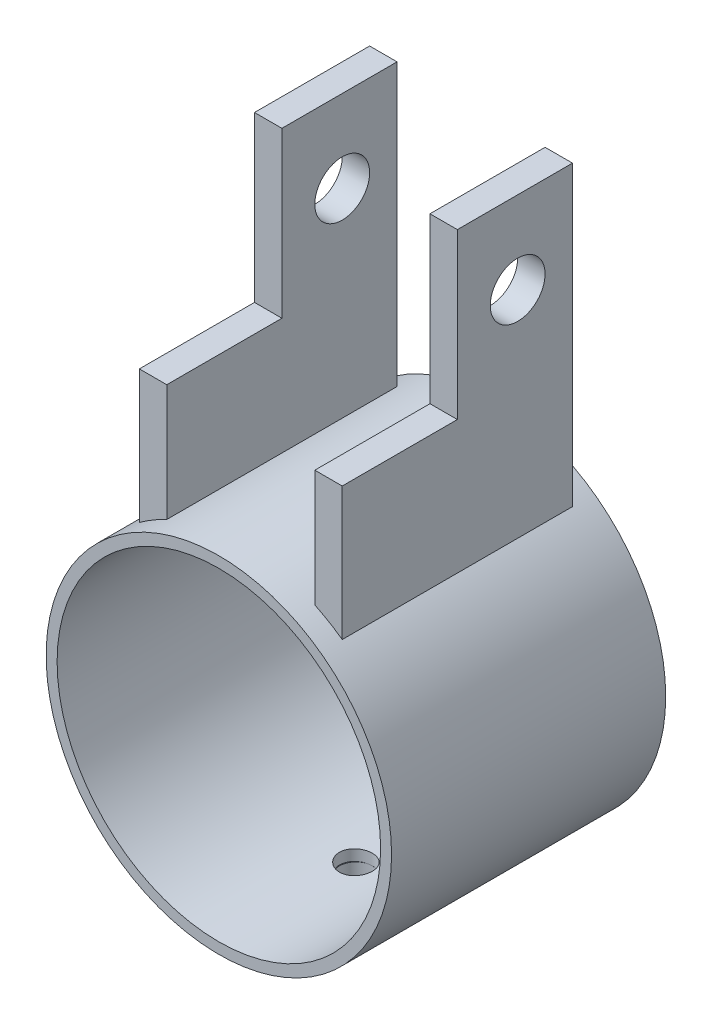
from build123d import *

# Parameters (mm, degrees)
SKETCH1_R                       = 31.5
SKETCH1_R_2                     = 29.5
BOSS_EXTRUDE1_DEPTH             = 50
BOSS_EXTRUDE2_REACH             = 102.468
BOSS_EXTRUDE2_END_RADIUS        = 31.5
SKETCH2_W                       = 5
SKETCH2_H                       = 42
BOSS_EXTRUDE2_DIRECTION_2_DEPTH = 30
SKETCH4_W                       = 21
SKETCH4_H                       = 30
CUT_EXTRUDE1_DEPTH              = 50
SKETCH5_R                       = 5
CUT_EXTRUDE2_DEPTH              = 50
SKETCH6_R                       = 3
CUT_EXTRUDE3_DEPTH              = 55
SKETCH7_R                       = 3
BOSS_EXTRUDE3_DEPTH             = 4


with BuildPart() as part:
    # Sketch1 → Boss-Extrude1 (new body)
    with BuildSketch(Plane.XY):
        Circle(SKETCH1_R)
        Circle(SKETCH1_R_2, mode=Mode.SUBTRACT)
    extrude(amount=BOSS_EXTRUDE1_DEPTH)

    # Boss-Extrude2: up to this cylinder (the profile starts outside it)
    boss_extrude2_end = Plane(origin=(0, 0, 25), z_dir=(0, 0, -1)) * Cylinder(BOSS_EXTRUDE2_END_RADIUS, 268.936, mode=Mode.PRIVATE)
    # Sketch2 → Boss-Extrude2 (add, up to the surface)
    with BuildSketch(Plane(origin=(0, 49.74998211, 0), x_dir=(1, 0, 0), z_dir=(0, 1, 0)), mode=Mode.PRIVATE) as boss_extrude2_sk1:
        with Locations((-16, -25)):
            Rectangle(SKETCH2_W, SKETCH2_H)
    boss_extrude2_tool1 = extrude(boss_extrude2_sk1.sketch, amount=-BOSS_EXTRUDE2_REACH, mode=Mode.PRIVATE) - boss_extrude2_end
    add(boss_extrude2_tool1.solids().sort_by_distance((-16, 49.749982, 25))[0])
    # Sketch2 → Boss-Extrude2 (add, up to the surface)
    with BuildSketch(Plane(origin=(0, 49.74998211, 0), x_dir=(1, 0, 0), z_dir=(0, 1, 0)), mode=Mode.PRIVATE) as boss_extrude2_sk2:
        with Locations((16, -25)):
            Rectangle(SKETCH2_W, SKETCH2_H)
    boss_extrude2_tool2 = extrude(boss_extrude2_sk2.sketch, amount=-BOSS_EXTRUDE2_REACH, mode=Mode.PRIVATE) - boss_extrude2_end
    add(boss_extrude2_tool2.solids().sort_by_distance((16, 49.749982, 25))[0])

    # Sketch2 → Boss-Extrude2 direction 2 (add)
    with BuildSketch(Plane(origin=(0, 49.74998211, 0), x_dir=(1, 0, 0), z_dir=(0, 1, 0))):
        with Locations((-16, -25)):
            Rectangle(SKETCH2_W, SKETCH2_H)
        with Locations((16, -25)):
            Rectangle(SKETCH2_W, SKETCH2_H)
    extrude(amount=BOSS_EXTRUDE2_DIRECTION_2_DEPTH)

    # Sketch4 → Cut-Extrude1 (cut)
    with BuildSketch(Plane.ZY.offset(18.5)):
        with Locations((35.5, 64.74998211)):
            Rectangle(SKETCH4_W, SKETCH4_H)
    extrude(amount=-CUT_EXTRUDE1_DEPTH, mode=Mode.SUBTRACT)

    # Sketch5 → Cut-Extrude2 (cut)
    with BuildSketch(Plane.ZY.offset(18.5)):
        with Locations((14, 64.74998211)):
            Circle(SKETCH5_R)
    extrude(amount=-CUT_EXTRUDE2_DEPTH, mode=Mode.SUBTRACT)

    # Sketch6 → Cut-Extrude3 (cut)
    with BuildSketch(Plane(origin=(0, 0, 0), x_dir=(1, 0, 0), z_dir=(0, 1, 0))):
        with Locations(Location((0, -25, 0), (0, 0, 270))):
            Circle(SKETCH6_R)
    extrude(amount=-CUT_EXTRUDE3_DEPTH, mode=Mode.SUBTRACT)


with BuildPart() as body_2:
    # Sketch7 → Boss-Extrude3 (new body)
    with BuildSketch(Plane(origin=(0, -35.5, 0), x_dir=(1, 0, 0), z_dir=(0, 1, 0))):
        Polygon((-4.101426834, -29.063450659), (1.468338081, -30.583665159), (5.569764915, -26.5202145), (4.101426834, -20.936549341), (-1.468338081, -19.416334841), (-5.569764915, -23.4797855), align=None)
        with Locations(Location((0, -25, 0), (0, 0, 270))):
            Circle(SKETCH7_R, mode=Mode.SUBTRACT)
    extrude(amount=BOSS_EXTRUDE3_DEPTH)


solid = Compound([part.part, body_2.part])
